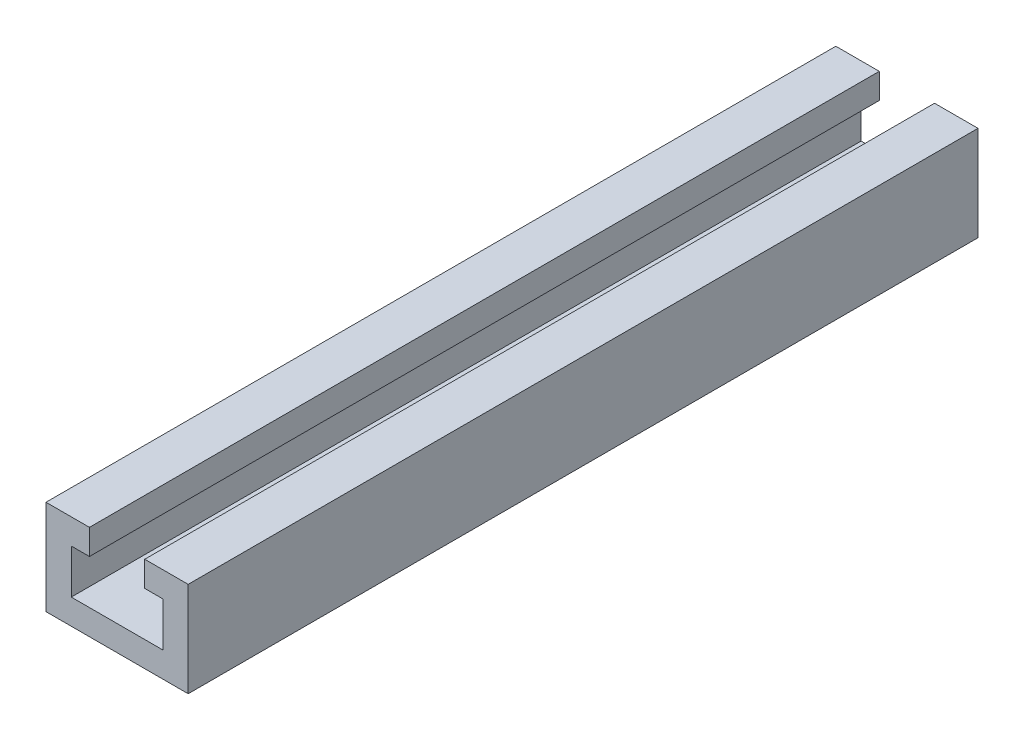
SolidWorks part; units mm, degrees
ref_plane "前视基准面" through (0, 0, 0) normal (0, 0, 1) x (1, 0, 0)
ref_plane "上视基准面" through (0, 0, 0) normal (0, 1, 0) x (1, 0, 0)
ref_plane "右视基准面" through (0, 0, 0) normal (1, 0, 0) x (0, 0, -1)
sketch "草图1" plane through (0, 0, 0) normal (0, 0, 1) x (1, 0, 0)
  line L0 (0, 0) -> (-4.5, 0)
  line L1 (-4.5, 0) -> (-4.5, 6)
  line L2 (-4.5, 6) -> (-1.75, 6)
  line L3 (-1.75, 6) -> (-1.75, 4.4)
  line L4 (-1.75, 4.4) -> (-2.9, 4.4)
  line L5 (-2.9, 4.4) -> (-2.9, 1.6)
  line L6 (-2.9, 1.6) -> (2.9, 1.6)
  line L7 (2.9, 1.6) -> (2.9, 4.4)
  line L8 (2.9, 4.4) -> (1.75, 4.4)
  line L9 (1.75, 4.4) -> (1.75, 6)
  line L10 (1.75, 6) -> (4.5, 6)
  line L11 (4.5, 6) -> (4.5, 0)
  line L12 (4.5, 0) -> (0, 0)
  dimension "D1" = 9
  dimension "D2" = 6
  dimension "D3" = 3.5
  dimension "D4" = 5.8
  dimension "D5" = 1.6
  dimension "D6" = 1.6
  dimension "D7" = 1.6
extrude "凸台-拉伸1" add sketch "草图1" along normal mid plane 50
